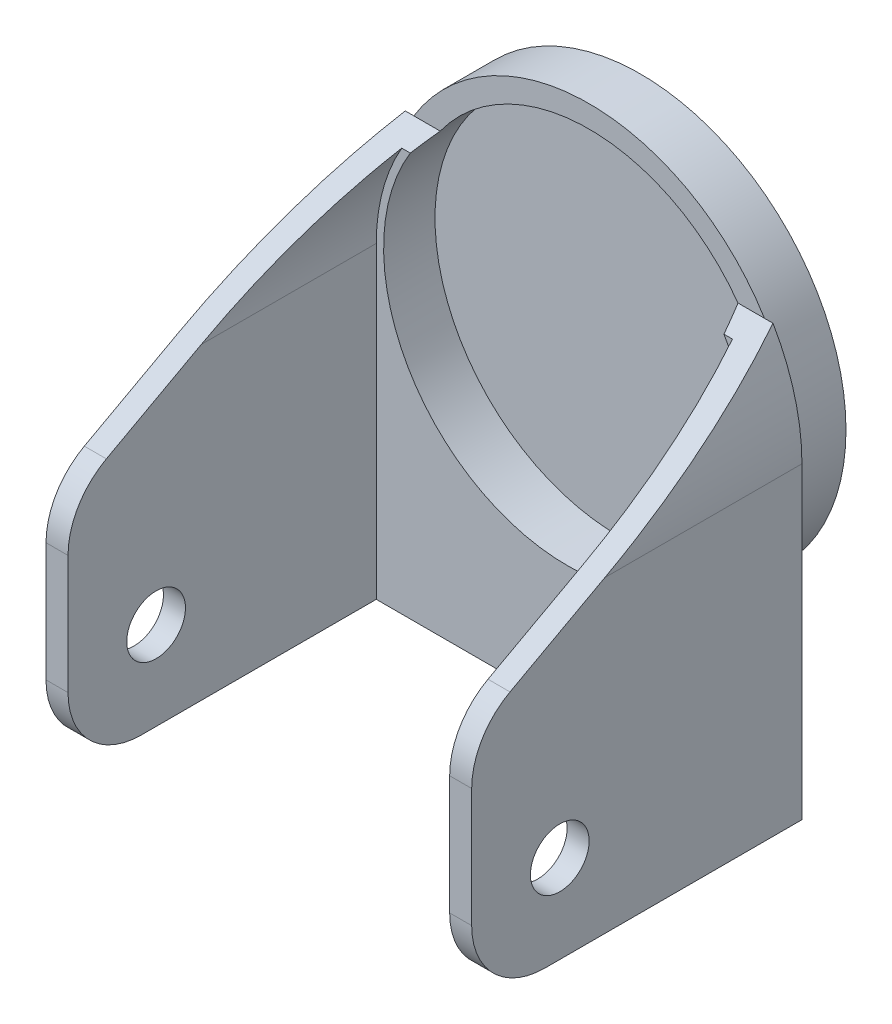
from build123d import *

# Parameters (mm, degrees)
SKETCH_1_R          = 12.5
EXTRUDE_1_DEPTH     = 3
SKETCH_2_R          = 28
EXTRUDE_2_DEPTH     = 10
SKETCH_3_R          = 25
CUT_EXTRUDE_1_DEPTH = 7
SKETCH_6_R          = 29
SKETCH_6_R_2        = 25
EXTRUDE_4_DEPTH     = 3
EXTRUDE_3_DEPTH     = 3
EXTRUDE_START       = 42
EXTRUDE_5_DEPTH     = 42
CUT_EXTRUDE_2_DEPTH = 91.293964361
FILLET_1_R          = 10
SKETCH_9_R          = 4
CUT_EXTRUDE_4_DEPTH = 91.293964361


with BuildPart() as part:
    # 草图1 → 凸台-拉伸1 (new body)
    with BuildSketch(Plane.XY):
        Circle(SKETCH_1_R)
    extrude(amount=EXTRUDE_1_DEPTH)

    # 草图2 → 凸台-拉伸2 (add)
    with BuildSketch(Plane.XY.offset(3)):
        Circle(SKETCH_2_R)
    extrude(amount=EXTRUDE_2_DEPTH)

    # 草图3 → 切除-拉伸1 (cut)
    with BuildSketch(Plane.XY.offset(13)):
        Circle(SKETCH_3_R)
    extrude(amount=-CUT_EXTRUDE_1_DEPTH, mode=Mode.SUBTRACT)

    # 草图6 → 凸台-拉伸4 (add)
    with BuildSketch(Plane.XY.offset(13)):
        Circle(SKETCH_6_R)
        Circle(SKETCH_6_R_2, mode=Mode.SUBTRACT)
    extrude(amount=-EXTRUDE_4_DEPTH)

    # 草图4 → 凸台-拉伸3 (add)
    with BuildSketch(Plane.XY.offset(13)):
        with BuildLine():
            ThreePointArc((29, 0), (0, -29), (-29, 0))
            Line((-29, 0), (-29, -42))
            Line((-29, -42), (29, -42))
            Line((29, -42), (29, 0))
        make_face()
    extrude(amount=-EXTRUDE_3_DEPTH)

    # 草图7 → 凸台-拉伸5 (add)
    with BuildSketch(Plane.XY.offset(13).offset(EXTRUDE_START)):
        with BuildLine():
            Line((-26, -42), (-26, 0))
            ThreePointArc((-26, 0), (0, 26), (26, 0))
            Line((26, 0), (26, -42))
            Line((26, -42), (29, -42))
            Line((29, -42), (29, 0))
            ThreePointArc((29, 0), (0, 29), (-29, 0))
            Line((-29, 0), (-29, -42))
            Line((-29, -42), (-26, -42))
        make_face()
    extrude(amount=-EXTRUDE_5_DEPTH)

    # 草图8 → 切除-拉伸2 (cut, through all)
    with BuildSketch(Plane(origin=(29, 0, 0), x_dir=(0, 0, -1), z_dir=(1, 0, 0))):
        Polygon((-55, -9.872511864), (-10, 14.609708665), (-10, 29), (-55, 29), align=None)
    extrude(amount=-CUT_EXTRUDE_2_DEPTH, mode=Mode.SUBTRACT)

    # 圆角1
    fillet_1_edges = [part.edges().sort_by_distance(p)[0] for p in [
        (27.5, -9.872511864, 55),
        (27.5, -42, 55),
        (-27.5, -9.872511864, 55),
        (-27.5, -42, 55),
    ]]
    fillet(fillet_1_edges, radius=FILLET_1_R)

    # 草图9 → 切除-拉伸4 (cut, through all)
    with BuildSketch(Plane(origin=(29, 0, 0), x_dir=(0, 0, -1), z_dir=(1, 0, 0))):
        with Locations(Location((-43, -30, 0), (0, 0, 90))):
            Circle(SKETCH_9_R)
    extrude(amount=-CUT_EXTRUDE_4_DEPTH, mode=Mode.SUBTRACT)


solid = part.part
